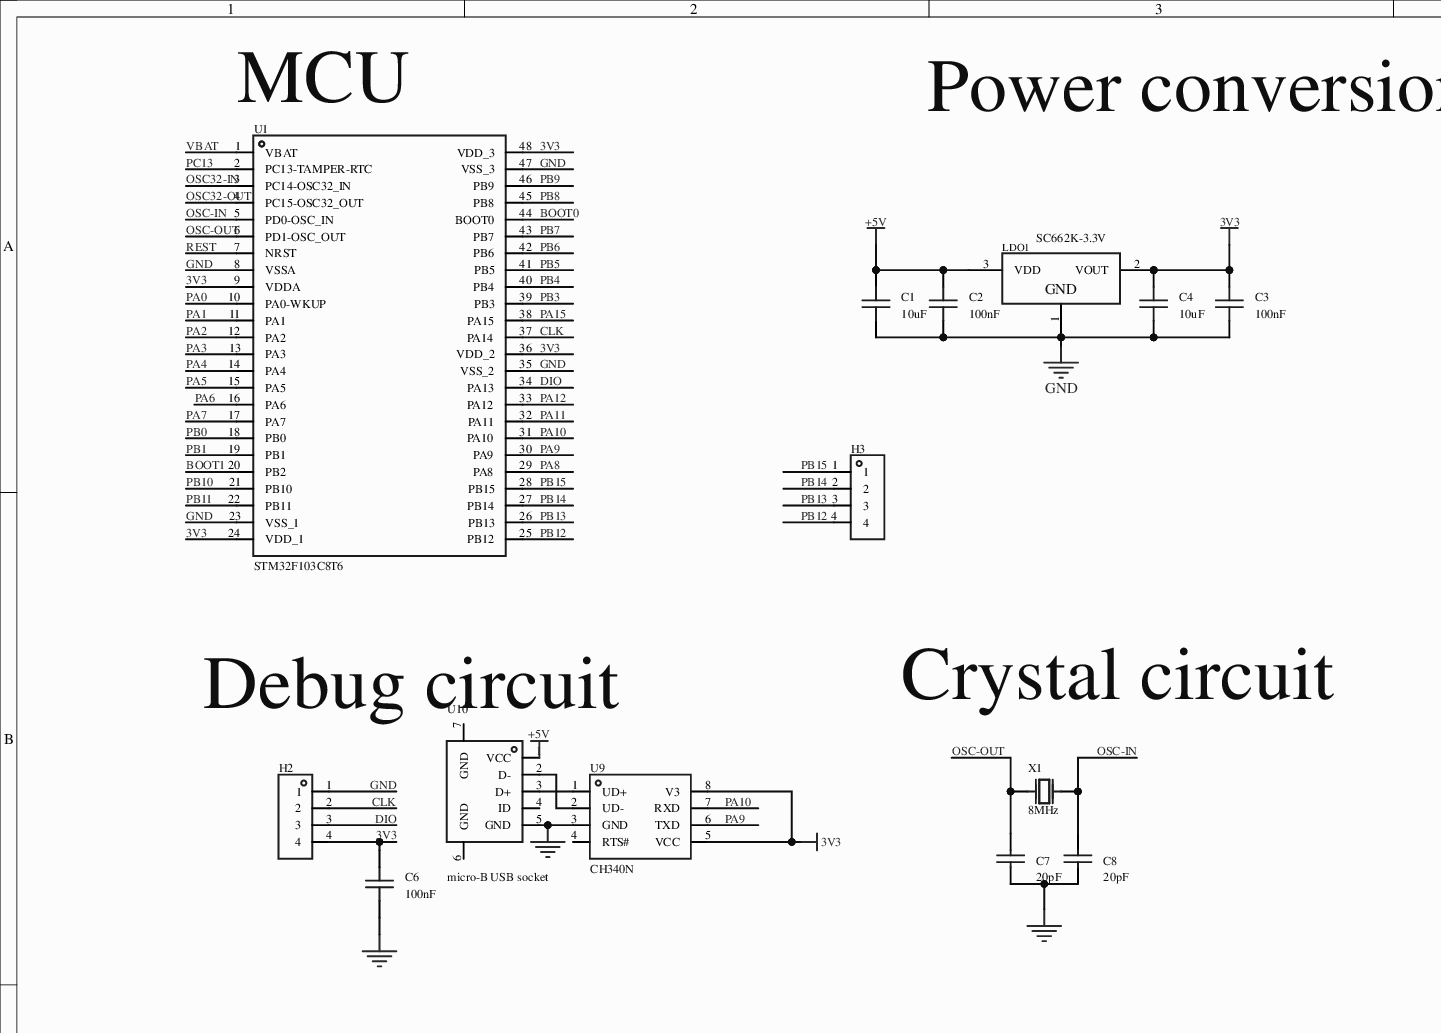
[diagram p0: MISC64779-3.schdoc, top left]
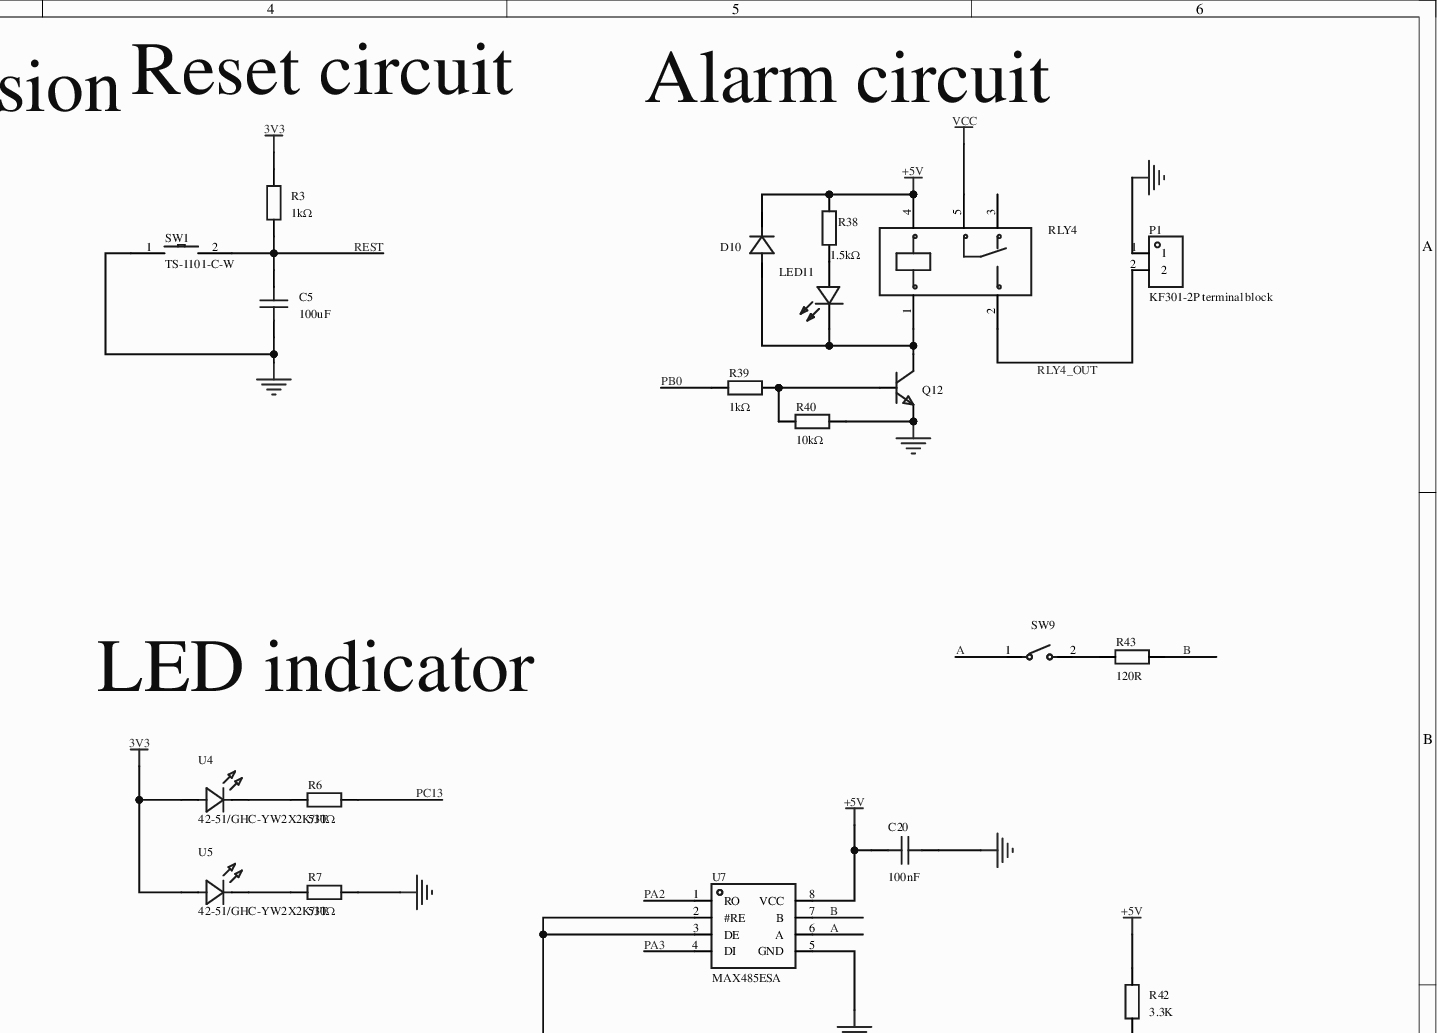
[diagram p1: MISC64779-3.schdoc, top right]
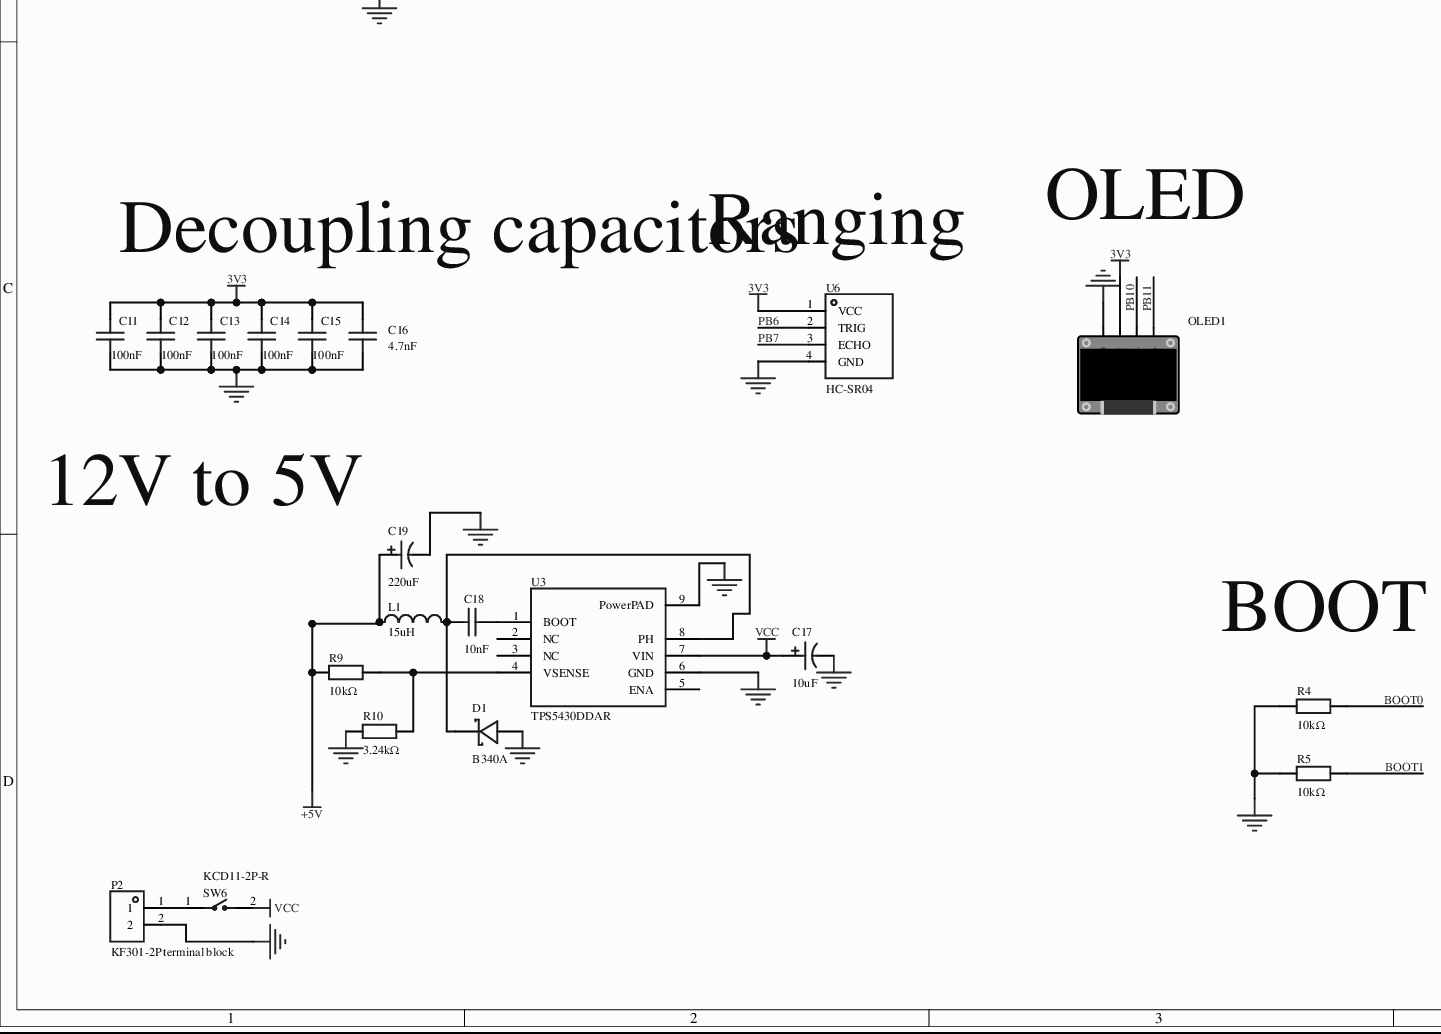
[diagram p2: MISC64779-3.schdoc, bottom left]
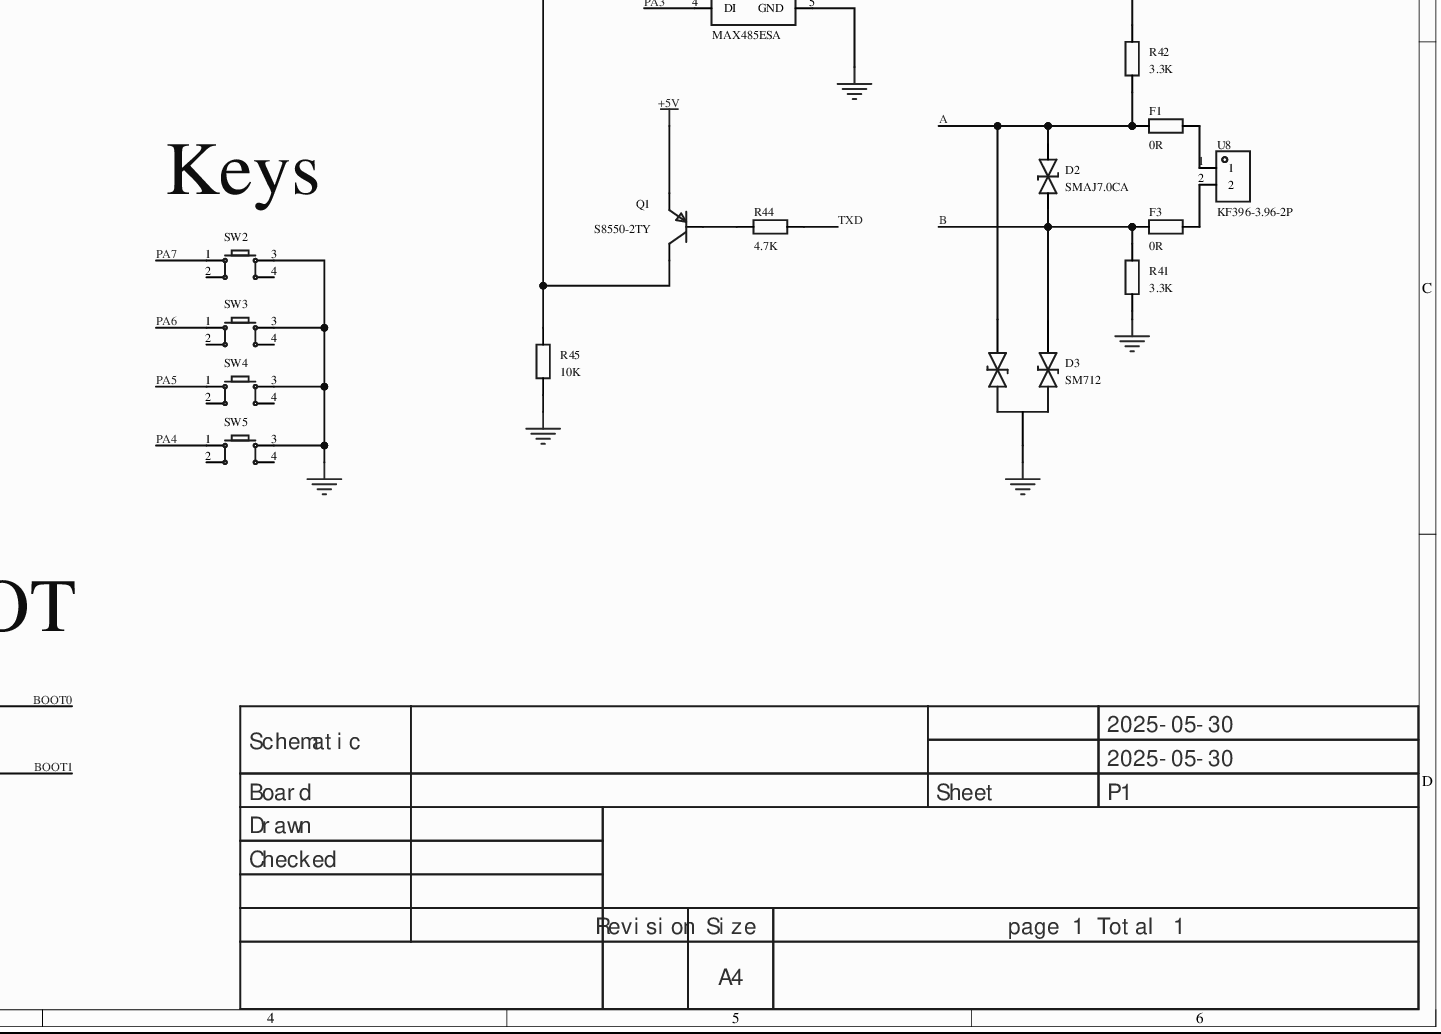
[diagram p3: MISC64779-3.schdoc, bottom right]
# Altium project MISC64779-2.PrjPcb
1 sheet, 67 parts. Net scope: global (net labels, ports and power ports of the same name join across sheets).
Board file: MISC64779.pcbdoc

## Sheet MISC64779-3.schdoc
size 420 x 297 mm; Version: V1.0; @Project Name: MISC64779; @Page Count: 1; @Update Date: 2025-05-30; @Create Date: 2025-05-30; @Schematic Name: MISC64779; @Page No: 1; @Create Time: 10:06:22; @Update Time: 12:30:53; @Board Name: MISC64779

### Parts
C1  10uF  [C0603]
C2  100nF  [C0603]
C3  100nF  [C0603]
C4  10uF  [C0603]
C5  100uF  [C1206]
C6  100nF  [C0603]
C7  20pF  [C0603]
C8  20pF  [C0603]
C11  100nF  [C0603]
C12  100nF  [C0603]
C13  100nF  [C0603]
C14  100nF  [C0603]
C15  100nF  [C0603]
C16  4.7nF  [C0603]
C17  10uF  [CAP-TH_BD5.0-P2.00-D0.8-FD]
C18  10nF  [C0603]
C19  220uF  [CAP-TH_BD6.3-P2.50-D1.0-FD]
C20  100nF  [C0603]
D1  B340A  [SMA_L4.3-W2.6-LS5.1-RD]
D2  SMAJ7.0CA  [SMA_L4.5-W2.7-LS5.1-BI]
D3  SM712  [SOT-23-3_L2.9-W1.3-P1.90-LS2.4-BR]
D10  1N4007  [SMA_L4.3-W2.5-LS5.0-RD]  (value not drawn)
F1  0R  [R0805]
F3  0R  [R0805]
H2  (no value)  [HDR-TH_4P-P2.54-V-M]
H3  (no value)  [HDR-TH_4P-P2.54-V-M]
L1  15uH  [IND-SMD_L7.0-W6.6_FXL0630]
LDO1  SC662K-3.3V  [SOT-23-3_L2.9-W1.3-P1.90-LS2.4-BR]
LED11  NCD0805R1  [LED0805-R-RD]  (value not drawn)
OLED1  (no value)  [0.96OLED_4P]
P1  KF301-2P terminal block  [CONN-TH_XY301V-A-5.0-2P]
P2  KF301-2P terminal block  [CONN-TH_XY301V-A-5.0-2P]
Q1  S8550-2TY  [SOT-23-3_L2.9-W1.3-P0.95-LS2.4-BR]
Q12  S8050 J3Y(RANGE:200-350)  [SOT-23-3_L3.0-W1.7-P0.95-LS2.9-BR]  (value not drawn)
R3  1kΩ  [R0603]
R4  10kΩ  [R0603]
R5  10kΩ  [R0603]
R6  510Ω  [R0603]
R7  510Ω  [R0603]
R9  10kΩ  [R0603]
R10  3.24kΩ  [R0603]
R38  1.5kΩ  [R0805]
R39  1kΩ  [R0805]
R40  10kΩ  [R0805]
R41  3.3K  [R0603]
R42  3.3K  [R0603]
R43  120R  [R0603]
R44  4.7K  [R0603]
R45  10K  [R0603]
RLY4  SRD-05VDC-SL-C  [RELAY-TH_SRD-XXVDC-XL-C]  (value not drawn)
SW1  TS-1101-C-W  [SW-SMD_L6.0-W3.3-LS8.0]
SW2  (no value)  [SW-TH_4P-L6.0-W6.0-P4.50-LS6.5]
SW3  (no value)  [SW-TH_4P-L6.0-W6.0-P4.50-LS6.5]
SW4  (no value)  [SW-TH_4P-L6.0-W6.0-P4.50-LS6.5]
SW5  (no value)  [SW-TH_4P-L6.0-W6.0-P4.50-LS6.5]
SW6  KCD11-2P-R  [SW-TH_2P-L15.0-W10.5-P5.00_KCD11-2P-R]
SW9  ZX-1.27BM-1PSMD  [SW-SMD_L5.4-W2.8-LS8.2]  (value not drawn)
U1  STM32F103C8T6  [LQFP-48_L7.0-W7.0-P0.50-LS9.0-BL]
U3  TPS5430DDAR  [ESOP-8_L4.9-W3.9-P1.27-LS6.0-TL-EP]
U4  42-51/GHC-YW2X2K/3T  [LED-SMD_L1.6-W0.8-FD_GREEN-1]
U5  42-51/GHC-YW2X2K/3T  [LED-SMD_L1.6-W0.8-FD_GREEN-1]
U6  HC-SR04  [TH_HC-SR04V]
U7  MAX485ESA  [SOP-8_L5.0-W4.0-P1.27-LS6.0-BL]
U8  KF396-3.96-2P  [CONN-TH_P3.96_KF396-3.96-2P]
U9  CH340N  [SOP-8_L4.9-W3.9-P1.27-LS6.0-BL]
U10  micro-B USB socket  [MICRO-USB_C9900039549]
X1  8MHz  [OSC-TH_L10.0-W4.5-P5.00]

### Nets
3V3: C3.2 C4.2 C6.2 C11.2 C12.2 C13.2 C14.2 C15.2 C16.2 H2.4 LDO1.2(VOUT) OLED1.2(VCC) R3.2 U1.9(VDDA) U1.24(VDD_1) U1.36(VDD_2) U1.48(VDD_3) U4.1(A) U5.1(A) U6.1(VCC) U9.5(VCC) U9.8(V3)
+5V: C1.2 C2.2 C19.1 C20.1 D10.1(K) L1.1 LDO1.3(VDD) Q1.2(E) R9.1 R38.2 R42.2 RLY4.4 U7.8(VCC) U10.1(VCC)
GND: C1.1 C2.1 C3.1 C4.1 C5.1 C6.1 C7.1 C8.1 C11.1 C12.1 C13.1 C14.1 C15.1 C16.1 C17.2 C19.2 C20.2 D1.2(A) D3.3 H2.1 LDO1.1(GND) OLED1.1(GND) P1.1 P2.2 Q12.2(E) R4.1 R5.1 R7.2 R10.1 R40.1 R41.1 R45.2 SW1.1 SW2.3 SW3.3 SW4.3 SW5.3 U1.8(VSSA) U1.23(VSS_1) U1.35(VSS_2) U1.47(VSS_3) U3.6(GND) U3.9(PowerPAD) U6.4(GND) U7.5(GND) U9.3(GND) U10.5(GND)
VCC: C17.1 RLY4.5 SW6.2 U3.7(VIN)
A: D2.2 D3.2 F1.1 R42.1 SW9.1 U7.6(A)
B: D2.1 D3.1 F3.1 R41.2 R43.2 U7.7(B)
BOOT0: R4.2 U1.44(BOOT0)
BOOT1: R5.2 U1.20(PB2)
CLK: H2.2 U1.37(PA14)
DIO: H2.3 U1.34(PA13)
OSC32-IN: U1.3(PC14-OSC32_IN)
OSC32-OUT: U1.4(PC15-OSC32_OUT)
OSC-IN: C8.2 U1.5(PD0-OSC_IN) X1.1(OSC1)
OSC-OUT: C7.2 U1.6(PD1-OSC_OUT) X1.2(OSC2)
PA0: U1.10(PA0-WKUP)
PA1: U1.11(PA1)
PA2: U1.12(PA2) U7.1(RO)
PA3: U1.13(PA3) U7.4(DI)
PA4: SW5.1 U1.14(PA4)
PA5: SW4.1 U1.15(PA5)
PA6: SW3.1 U1.16(PA6)
PA7: SW2.1 U1.17(PA7)
PA8: U1.29(PA8)
PA9: U1.30(PA9) U9.6(TXD)
PA10: U1.31(PA10) U9.7(RXD)
PA11: U1.32(PA11)
PA12: U1.33(PA12)
PA15: U1.38(PA15)
PB0: R39.1 U1.18(PB0)
PB1: U1.19(PB1)
PB3: U1.39(PB3)
PB4: U1.40(PB4)
PB5: U1.41(PB5)
PB6: U1.42(PB6) U6.2(TRIG)
PB7: U1.43(PB7) U6.3(ECHO)
PB8: U1.45(PB8)
PB9: U1.46(PB9)
PB10: OLED1.3(SCL) U1.21(PB10)
PB11: OLED1.4(SDA) U1.22(PB11)
PB12: H3.4 U1.25(PB12)
PB13: H3.3 U1.26(PB13)
PB14: H3.2 U1.27(PB14)
PB15: H3.1 U1.28(PB15)
PC13: R6.2 U1.2(PC13-TAMPER-RTC)
REST: C5.2 R3.1 SW1.2 U1.7(NRST)
RLY4_OUT: P1.2 RLY4.2
TXD: R44.1
VBAT: U1.1(VBAT)
NetC18_1: C18.1 D1.1(K) L1.2 U3.8(PH)
NetC18_2: C18.2 U3.1(BOOT)
NetD10_2: D10.2(A) LED11.2(-) Q12.3(C) RLY4.1
NetF1_2: F1.2 U8.1
NetF3_2: F3.2 U8.2
NetLED11_1: LED11.1(+) R38.1
NetP2_1: P2.1 SW6.1
NetQ1_1: Q1.1(B) R44.2
NetQ1_3: Q1.3(C) R45.1 U7.2(#RE) U7.3(DE)
NetQ12_1: Q12.1(B) R39.2 R40.2
NetR6_1: R6.1 U4.2(C)
NetR7_1: R7.1 U5.2(C)
NetR9_2: R9.2 R10.2 U3.4(VSENSE)
NetR43_1: R43.1 SW9.2
NetU9_1: U9.1(UD+) U10.3(D+)
NetU9_2: U9.2(UD-) U10.2(D-)

Not connected (* = marked no-connect by the designer): RLY4 3*; SW2 2 4; SW3 2 4; SW4 2 4; SW5 2 4; U3 2(NC) 3(NC) 5(ENA); U9 4(RTS#); U10 4(ID) 6(GND) 7(GND)

### Notes on the sheet
- (near U1) MCU
- Power conversion
- Reset circuit
- Alarm circuit
- 供电用12v供电
  有超声波测距功能
  具备连接上位机的功能
  有报警功能（留接口）
  用户按键，LED
  温湿度，oled显示
- (near U10) Debug circuit
- Crystal circuit
- LED indicator
- (near SW2) Keys
- Decoupling capacitors
- (near U6) Ranging
- OLED
- (near C19) 12V to 5V
- (near R4) BOOT
- 2025-05-30
- Schematic
- Board
- Sheet
- P1
- Drawn
- Checked
- Revision
- Size
- A4
- page 1 Total 1

### Library data of the parts
C1 C4 = CL10A106KP8NNNC: Capacitance:10uF;Tolerance:±10%;Rated voltage:10V;Dielectric (temp. coefficient):X5R;; Manufacturer: SAMSUNG(三星); AddInBom: yes; ModelId: ac125912035d415993ca9572d50418b1; ModelName: C0603_L1.6-W0.8-H0.8; ModelTransform: 62.992,31.496,0,0,0,0,0,0,0; Tolerance: ±10%; Voltage Rated: 10V; Temperature Coefficient: X5R; Device: CL10A106KP8NNNC; Symbol: CL10A106KP8NNNC; LCSC Part Name: 10uF ±10% 10V; SupplierPart: C19702; ManufacturerPart: CL10A106KP8NNNC; Supplier Footprint: 0603; JLCPCB Part Class: Basic library; Datasheet: example.com/20160103/1457707703378.pdf; Supplier: LCSC; ConvertToPcb: yes; FootprintName: C0603; Value: 10uF
C2 C3 = CC0603KRX7R9BB104: Capacitance:100nF;Tolerance:±10%;Rated voltage:50V;Dielectric (temp. coefficient):X7R;; Manufacturer: YAGEO(国巨); AddInBom: yes; ModelId: ac125912035d415993ca9572d50418b1; ModelName: C0603_L1.6-W0.8-H0.8; ModelTransform: 62.992,31.496,0,0,0,0,0,0,0; Tolerance: ±10%; Voltage Rated: 50V; Temperature Coefficient: X7R; Device: CC0603KRX7R9BB104; Symbol: CC0603KRX7R9BB104; LCSC Part Name: 100nF ±10% 50V; SupplierPart: C14663; ManufacturerPart: CC0603KRX7R9BB104; Supplier Footprint: 0603; JLCPCB Part Class: Basic library; Datasheet: example.com/20180910/C282072_33301C7F631E79921B82A8DAC6BCC5B3.pdf; Supplier: LCSC; ConvertToPcb: yes; FootprintName: C0603; Value: 100nF
C5 = HGC1206R5107M100NSPJ: Capacitance:100uF;Tolerance:±20%;Rated voltage:10V;Dielectric (temp. coefficient):X5R;; Manufacturer: Chinocera(华瓷); AddInBom: yes; ModelId: e4be705b945545a48e666415e3682bd8; ModelName: C1206_L3.2-W1.6-H1.3; ModelTransform: 125.984,62.992,0,0,0,0,0,0,0; Tolerance: ±20%; Voltage Rated: 10V; Temperature Coefficient: X5R; Symbol: HGC1206R5107M100NSPJ; Device: HGC1206R5107M100NSPJ; LCSC Part Name: 100uF ±20% 10V; SupplierPart: C7432784; ManufacturerPart: HGC1206R5107M100NSPJ; Supplier Footprint: 1206; JLCPCB Part Class: Extended library; Datasheet: example.com/20240320/FAC3FEC40A78BC5CCCE96C232A94D860.pdf; Supplier: LCSC; ConvertToPcb: yes; FootprintName: C1206; Value: 100uF
C6 C11-C15 = CGA0603X7R104K500JT: Capacitance:100nF;Tolerance:±10%;Rated voltage:50V;Dielectric (temp. coefficient):X7R;; Manufacturer: HRE(芯声); AddInBom: yes; ModelId: ac125912035d415993ca9572d50418b1; ModelName: C0603_L1.6-W0.8-H0.8; ModelTransform: 62.992,31.496,0,0,0,0,0,0,0; Tolerance: ±10%; Voltage Rated: 50V; Temperature Coefficient: X7R; Symbol: CGA0603X7R104K500JT; Device: CGA0603X7R104K500JT; LCSC Part Name: 100nF ±10% 50V; SupplierPart: C6119867; ManufacturerPart: CGA0603X7R104K500JT; Supplier Footprint: 0603; JLCPCB Part Class: Extended library; Supplier: LCSC; ConvertToPcb: yes; FootprintName: C0603; Value: 100nF
C7 C8 = CL10C200JB8NNNC: Capacitance:20pF;Tolerance:±5%;Rated voltage:50V;Dielectric (temp. coefficient):C0G;; Manufacturer: SAMSUNG(三星); AddInBom: yes; ModelId: ac125912035d415993ca9572d50418b1; ModelName: C0603_L1.6-W0.8-H0.8; ModelTransform: 62.992,31.496,0,0,0,0,0,0,0; Tolerance: ±5%; Voltage Rated: 50V; Temperature Coefficient: C0G; Symbol: CL10C200JB8NNNC; Device: CL10C200JB8NNNC; LCSC Part Name: 20pF ±5% 50V; SupplierPart: C1648; ManufacturerPart: CL10C200JB8NNNC; Supplier Footprint: 0603; JLCPCB Part Class: Basic library; Datasheet: example.com/20160218/1457707763339.pdf; Supplier: LCSC; ConvertToPcb: yes; FootprintName: C0603; Value: 20pF
C16 = CGA0603X7R472K500JT: Capacitance:4.7nF;Tolerance:±10%;Rated voltage:50V;Dielectric (temp. coefficient):X7R;; Manufacturer: HRE(芯声); AddInBom: yes; ModelId: ac125912035d415993ca9572d50418b1; ModelName: C0603_L1.6-W0.8-H0.8; ModelTransform: 62.992,31.496,0,0,0,0,0,0,0; Tolerance: ±10%; Voltage Rated: 50V; Temperature Coefficient: X7R; Symbol: CGA0603X7R472K500JT; Device: CGA0603X7R472K500JT; LCSC Part Name: 4.7nF ±10% 50V; SupplierPart: C7503499; ManufacturerPart: CGA0603X7R472K500JT; Supplier Footprint: 0603; JLCPCB Part Class: Extended library; Supplier: LCSC; ConvertToPcb: yes; FootprintName: C0603; Value: 4.7nF
C17 = KM106M050D11RR0VH2FP0: Capacitance:10uF;Tolerance:±20%;Rated voltage:50V;; Manufacturer: CX(承兴); Symbol: 10uF 50V 5*11; AddInBom: yes; ModelId: edeeed87cbc746108d01291548c38636; ModelName: CAP-TH_D5.0×H7.0×P2.0; ModelTransform: 197.091,196.7911,0,0,0,0,0,0,-137.795; Tolerance: ±20%; Rated Voltage: 50V; φD: 5mm; L: 11mm; Lifetime @ Temp: 1000hrs@105℃; Device: KM106M050D11RR0VH2FP0; Supplier: LCSC; Manufacturer Part: KM106M050D11RR0VH2FP0; Value: 10uF; Supplier Part: C43345; JLCPCB Part Class: Extended library; LCSC Part Name: 10uF ±20% 50V; Supplier Footprint: 插件,D5xL11mm; Datasheet: example.com/20211027/06D6BA3719C264B639DC286D935D03EA.pdf; ConvertToPcb: yes; FootprintName: CAP-TH_BD5.0-P2.00-D0.8-FD; Lead Spacing: 2mm
C18 = CC0603KRX7R9BB103: Capacitance:10nF;Tolerance:±10%;Rated voltage:50V;Dielectric (temp. coefficient):X7R;; Manufacturer: YAGEO(国巨); AddInBom: yes; ModelId: ac125912035d415993ca9572d50418b1; ModelName: C0603_L1.6-W0.8-H0.8; ModelTransform: 62.992,31.496,0,0,0,0,0,0,0; Tolerance: ±10%; Voltage Rated: 50V; Temperature Coefficient: X7R; Symbol: CC0603KRX7R9BB103; Device: CC0603KRX7R9BB103; Supplier: LCSC; Manufacturer Part: CC0603KRX7R9BB103; Value: 10nF; Supplier Part: C100042; JLCPCB Part Class: Extended library; LCSC Part Name: 10nF ±10% 50V; Supplier Footprint: 0603; Datasheet: example.com/20181008/C309510_22F155564471FAF6A489F7D68F34234E.pdf; ConvertToPcb: yes; FootprintName: C0603
C19 = KM227M016E11RR0VH2FP0: Capacitance:220uF;Tolerance:±20%;Rated voltage:16V;Ripple current:-;Equivalent series resistance:-;; Manufacturer: CX(承兴); Symbol: 220uF 16V 6.3*11; AddInBom: yes; ModelId: 0a4db4bf24b443b3be4905be97ff10c5; ModelTransform: 248.4247,247.99777,0,0,0,0,0,0,-137.795; Tolerance: ±20%; Rated Voltage: 16V; φD: 6.3mm; L: 11mm; Lifetime @ Temp: 1000hrs@105℃; Device: KM227M016E11RR0VH2FP0; Supplier: LCSC; Manufacturer Part: KM227M016E11RR0VH2FP0; Value: 220uF; Supplier Part: C43349; JLCPCB Part Class: Extended library; LCSC Part Name: 220uF ±20% 16V; Supplier Footprint: 插件,D6.3xL11mm; Datasheet: example.com/20211027/06D6BA3719C264B639DC286D935D03EA.pdf; ConvertToPcb: yes; FootprintName: CAP-TH_BD6.3-P2.50-D1.0-FD; ModelName: CAP-TH_BD6.3-P2.50-D1.0-FD; Ripple Current: -; Equivalent Series Resistance(ESR): -; Lead Spacing: 2.5mm
C20 = CAP_0603: ConvertToPcb: yes; SymbolName: CapAcitance; ModelId: ac125912035d415993ca9572d50418b1; ModelName: C0603_L1.6-W0.8-H0.8; ModelTransform: 62.992,31.496,0,0,0,0,0,0,0; Device: CAP_0603; AddInBom: yes; Supplier Footprint: 0603; FootprintName: C0603; Value: 100nF
D1 = B340A: Forward voltage drop (Vf):550mV@3A;DC reverse voltage (Vr):40V;Average rectified current (Io):3A;; Manufacturer: MDD; AddInBom: yes; ModelId: 1d20a911e9694ba6aaf6e9207164e4da; ModelTransform: 196.4563,102.362,0,0,0,0,0,0,0; Reverse Voltage (Vr): 40V; Average Rectified Current (Io): 3A; Symbol: B340A; Device: B340A; Supplier: LCSC; Manufacturer Part: B340A; Supplier Part: C64982; JLCPCB Part Class: Extended library; LCSC Part Name: 电压:40V 电流:3A; Supplier Footprint: SMA(DO-214AC); Datasheet: example.com/20230710/CC7CF81239BC87A7012E02A96905E83C.pdf; ConvertToPcb: yes; FootprintName: SMA_L4.3-W2.6-LS5.1-RD; ModelName: SMA_L4.3-W2.6-LS5.1-RD; Forward Voltage (Vf@If): 550mV@3A
D2 = SMAJ7.0CA_C383701: Reverse standoff voltage (Vrwm):7V;Max clamping voltage:12V;Peak pulse current (Ipp)@10/1000us:33.3A;Breakdown voltage:7.78V;; Manufacturer: BORN(伯恩半导体); AddInBom: yes; ModelId: c57f874422f846fca512c5458c0e414d; ModelTransform: 200.787,106.299,0,0,0,0,0,0,0; Reverse Stand-Off Voltage (Vrwm): 7V; Maximum Clamping Voltage: 12V; Peak Pulse Current (Ipp)@10/1000us: 33.3A; Breakdown Voltage: 7.78V; Type: TVS; Symbol: SMAJ7.0CA_C383701; Device: SMAJ7.0CA_C383701; Supplier: LCSC; Supplier Part: C383701; Manufacturer Part: SMAJ7.0CA; JLCPCB Part Class: Extended library; LCSC Part Name: SMAJ7.0CA; Supplier Footprint: SMA(DO-214AC); Datasheet: example.com/20190401/C383701_4E66D368F6F089B11959B32E4033EF5C.pdf; ConvertToPcb: yes; FootprintName: SMA_L4.5-W2.7-LS5.1-BI; ModelName: SMA_L4.5-W2.7-LS5.1-BI
D3 = SM712_C521963: eak Pulse Current ( tp =8/20μs ) (note1) IPP 17A，反向截断电压VRWM 7V+12V 反向漏泄电流IR=1μA，VC12V 17A=26V VC7V 17A=12V 结电容75PF; Manufacturer: TECH PUBLIC(台舟); AddInBom: yes; ModelId: c62791f0466c4ae2a892c056b845b0ca; ModelName: SOT-23-3P_L2.9-W1.3-H1.0-LS2.4-P0.95; ModelTransform: 98.425,114.173,0,180,0,0,0.0005,-0.0005,0; Symbol: SM712_C521963; Device: SM712_C521963; Supplier: LCSC; Supplier Part: C521963; Manufacturer Part: SM712; JLCPCB Part Class: Extended library; LCSC Part Name: SM712; Supplier Footprint: SOT-23; Datasheet: example.com/20210810/E76C7C1824B0CB2A5B8963B3ABCE2DCE.pdf; ConvertToPcb: yes; FootprintName: SOT-23-3_L2.9-W1.3-P1.90-LS2.4-BR
D10 = 1N4007_C727081: Diode configuration:Single;Forward voltage drop (Vf):1.1V@1A;DC reverse voltage (Vr):1kV;Rectified current:1A;; Manufacturer: TWGMC(台湾迪嘉); AddInBom: yes; ModelId: 5b53cc1b87a148cc9fa13125be89f948; ModelTransform: 194.8815,98.425,0,0,0,0,0,0,0; Diode Configuration: Single; Reverse Voltage (Vr): 1kV; Rectified Current: 1A; Reverse Leakage Current (Ir): 5uA; Symbol: 1N4007_C727081; Device: 1N4007_C727081; LCSC Part Name: 1N4007; SupplierPart: C727081; ManufacturerPart: 1N4007; Supplier Footprint: SMA(DO-214AC); JLCPCB Part Class: Extended library; Datasheet: example.com/20200828/C727079_3A05254382567072883400655AE0ED46.pdf; Supplier: LCSC; ConvertToPcb: yes; FootprintName: SMA_L4.3-W2.5-LS5.0-RD; ModelName: SMA_L4.3-W2.5-LS5.0-RD; Forward Voltage (Vf@If): 1.1V@1A
F1 F3 = Res_0805: Symbol: Resistor; ConvertToPcb: yes; ModelId: 37a81e68749a4138bd2dfa6897b24b85; ModelName: R0805_L2.0-W1.3-H0.6; ModelTransform: 78.74,51.181,0,0,0,0,0,-0.0005,0; Value: 0R; Device: Res_0805; AddInBom: yes; Supplier Footprint: 0805; FootprintName: R0805
H2 H3 = HDR-M_2.54_1x4P: Symbol: PZ254V-11-04P; ConvertToPcb: yes; ModelId: 112f4d05e8d64e99ab9a333894bea4f9; ModelName: HDR-TH_4P-P2.54-M-LI-1X4P; ModelTransform: 399.999,104.7242,0,0,0,0,0,0,-118.11; Device: HDR-M_2.54_1x4P; AddInBom: yes; SupplierPart: C492403; Supplier Footprint: 插件; FootprintName: HDR-TH_4P-P2.54-V-M
L1 = FXL0630-150-M: Inductance:15uH;Tolerance:±20%;Rated current:3A;Saturation current (Isat):4.5A;Type:Integrally molded inductor;; Manufacturer: cjiang(长江微电); AddInBom: yes; ModelId: 6712504104d74f0ca01cd7d0df9965b7; ModelName: IND-SMD_L7.0-W6.6-H2.8_FXL0630; ModelTransform: 275.59,259.842,0,0,0,0,0,0,0; Tolerance: ±20%; Rated Current: 3A; Saturation Current (Isat): 4.5A; DC Resistance (DCR): 115mΩ; Symbol: FXL0630-150-M; Device: FXL0630-150-M; LCSC Part Name: 15uH ±20% 4.5A; SupplierPart: C177243; ManufacturerPart: FXL0630-150-M; Supplier Footprint: SMD,6.6x7mm; JLCPCB Part Class: Extended library; Datasheet: example.com/20230516/3A080F5AF8C87BB81C3BA86E5F60E51A.pdf; Supplier: LCSC; ConvertToPcb: yes; FootprintName: IND-SMD_L7.0-W6.6_FXL0630; Value: 15uH; Type: Integrally molded inductor
LDO1 = SC662K-3.3V: Output type:Fixed;Output polarity:Positive;Max input voltage:6V;Output voltage:3.3V;Output current:250mA;Power supply ripple rejection (PSRR):50dB@(1kHz);; Manufacturer: FM(富满); AddInBom: yes; ModelId: c62791f0466c4ae2a892c056b845b0ca; ModelName: SOT-23-3P_L2.9-W1.3-H1.0-LS2.4-P0.95; ModelTransform: 98.425,114.173,0,180,0,0,0.0005,-0.0005,0; Output Type: Fixed; Number of Outputs: 1; Maximum Input Voltage: 6V; Output Voltage: 3.3V; Dropout Voltage: 38mV@(10mA); Output Current: 250mA; Symbol: SC662K-3.3V; Device: SC662K-3.3V; Supplier: LCSC; Manufacturer Part: SC662K-3.3V; Supplier Part: C83932; JLCPCB Part Class: Extended library; LCSC Part Name: 输入6V 输出3.3V 250mA 停产; Supplier Footprint: SOT-23; Datasheet: example.com/20161024/1477288576049.pdf; ConvertToPcb: yes; FootprintName: SOT-23-3_L2.9-W1.3-P1.90-LS2.4-BR; Output Polarity: Positive; Power Supply Rejection Ratio (PSRR): 50dB@(1kHz)
LED11 = NCD0805R1: 灯头类型:-;发光颜色:红色;正向电压(VF):1.6V~2.6V;功率:65mW;正向电流:20mA;主波长:615nm~630nm;二极管配置:独立二极管;透镜颜色:无色透明透镜;色温:-;发光强度:67mcd~195mcd;发光角度:130°;载带方式:-;工作温度:-30℃~+85℃;; Manufacturer: 国星光电; Symbol: FC-2012HRK-620D; AddInBom: yes; ModelId: 6ccd75a2b5134d6ab756ecf3c14a7290; ModelName: LED0805-RD; ModelTransform: 79.527,49.2125,0,0,0,0,0,0,0; Emitted Color: Red; Power Dissipation: 65mW; Forward Current: 20mA; Diode Configuration: Single diode; Lens Color: Clear lens; Viewing Angle: 130°; Device: NCD0805R1; LCSC Part Name: NCD0805R1; SupplierPart: C84256; ManufacturerPart: NCD0805R1; Supplier Footprint: 0805; JLCPCB Part Class: Basic library; Datasheet: example.com/20200820/C84256_F0A75A43B3EAD75808600A0514C76B99.pdf; Supplier: LCSC; ConvertToPcb: yes; FootprintName: LED0805-R-RD; Lamp Holder Type: -; Forward Voltage (VF): 1.6V~2.6V; Dominant Wavelength: 615nm~630nm; Peak Wavelength: -; Color Temperature: -; Luminous Intensity: 67mcd~195mcd; Mounting Sytle: -; Operating Temperature: -30℃~+85℃
OLED1 = 0.96OLED模块_4P: Device: 0.96OLED module_4P; ConvertToPcb: yes; ModelId: 79c000fdb68d45a296c2e9bedf4f9055; ModelTransform: 1393.69792,1318.895,0,0,0,0,0,-560.079,-137.795; AddInBom: yes; SymbolName: 0.96OLED module_4P; FootprintName: 0.96OLED_4P; Supplier Footprint: 插件; ModelName: 0.96OLED_4P
P1 P2 = KF301-2P接线端子: AddInBom: yes; ModelId: ef7ead88b0f2448d904975b26718870f; ModelTransform: 417.322,299.212,0,0,0,0,11.811,-7.835,-157.48; Symbol: KF301-2P terminal block; Device: KF301-2P terminal block; LCSC Part Name: KF301-2P接线端子; SupplierPart: C9900016950; ManufacturerPart: KF301-2P接线端子; Supplier Footprint: CK301-2P; JLCPCB Part Class: Extended library; Supplier: LCSC; ConvertToPcb: yes; FootprintName: CONN-TH_XY301V-A-5.0-2P; ModelName: CONN-TH_XY301V-A-5.0-2P
Q1 = S8550-2TY: Transistor type:PNP;Collector current (Ic):1.5A;Collector-emitter breakdown voltage (Vceo):25V;Power (Pd):300mW;; Manufacturer: MDD; AddInBom: yes; ModelId: c62791f0466c4ae2a892c056b845b0ca; ModelName: SOT-23-3P_L2.9-W1.3-H1.0-LS2.4-P0.95; ModelTransform: 98.425,114.173,0,180,0,0,0.0005,-0.0005,0; Transistor Type: PNP; Collector Current (Ic): 1.5A; Collector-Emitter Breakdown Voltage (Vceo): 25V; Power Dissipation (Pd): 300mW; Transition Frequency (fT): 100MHz; Collector Cut-Off Current (Icbo): 100nA; Collector-Emitter Saturation Voltage (VCE(sat)@Ic,Ib): 500mV@800mA,80mA; Symbol: S8550-2TY; Device: S8550-2TY; Supplier: LCSC; Supplier Part: C364313; Manufacturer Part: S8550-2TY; JLCPCB Part Class: Extended library; LCSC Part Name: PNP 电流:1.5A 耐压:25V; Supplier Footprint: SOT-23; Datasheet: example.com/20230823/1A247BF48B2A25A14EBA2E9BB5B5D25C.pdf; ConvertToPcb: yes; FootprintName: SOT-23-3_L2.9-W1.3-P0.95-LS2.4-BR; Operating Temperature: -
Q12 = S8050 J3Y(RANGE:200-350): Transistor type:NPN;Collector current (Ic):500mA;Collector-emitter breakdown voltage (Vceo):25V;Power dissipation (Pd):300mW;DC current gain (hFE):200@500mA,1V;; Manufacturer: CJ(江苏长电/长晶); Symbol: S8050_C2146; AddInBom: yes; ModelId: 89cb27a44ab2466697082bb9fd73a7d0; ModelName: SOT-23-3L_L2.9-W1.6-H1.1-LS2.8-P0.95; ModelTransform: 114.173,110.236,0,90,0,0,0,0,0; type: NPN; Current - Collector(Ic): 500mA; Collector - Emitter Voltage VCEO: 25V; Pd - Power Dissipation: 300mW; Transition frequency(fT): 150MHz; Current - Collector Cutoff: 100nA; Vce Saturation(VCE(sat)): 600mV; Device: S8050 J3Y(RANGE:200-350); LCSC Part Name: H档(200-350); SupplierPart: C2146; ManufacturerPart: S8050 J3Y(RANGE:200-350); Supplier Footprint: SOT-23; JLCPCB Part Class: Basic library; Datasheet: example.com/20231013/FF37B6A000E6CDA75C9C999D2E78731F.pdf; Supplier: LCSC; ConvertToPcb: yes; FootprintName: SOT-23-3_L3.0-W1.7-P0.95-LS2.9-BR; DC Current Gain: 200@500mA,1V; Operating Temperature: -55℃~+150℃
R3 = RC0603FR-071KL: Resistor type:Thick-film resistor;Resistance:1kΩ;Tolerance:±1%;Power:100mW;Max working voltage:75V;Temperature coefficient:±100ppm/℃;; Manufacturer: YAGEO(国巨); AddInBom: yes; ModelId: fc143cca1e79419f9cd78b61e9279f08; ModelTransform: 31.8897,63.7794,0,90,0,0,0,0,0; Tolerance: ±1%; Power(Watts): 100mW; Overload Voltage (Max): 75V; Symbol: RC0603FR-071KL; Device: RC0603FR-071KL; LCSC Part Name: 厚膜电阻 1kΩ ±1% 100mW; SupplierPart: C22548; ManufacturerPart: RC0603FR-071KL; Supplier Footprint: 0603; JLCPCB Part Class: Extended library; Datasheet: example.com/20180316/70C0E2BDAE7FCC62C531A5A58D202EE1.pdf; Supplier: LCSC; ConvertToPcb: yes; FootprintName: R0603; ModelName: R0603; Type: Thick-film resistor; Value: 1kΩ; Temperature Coefficient: ±100ppm/℃; Operating Temperature Range: -55℃~+155℃
R4 R5 R9 = 0603WAF1002T5E: Resistor type:Thick-film resistor;Resistance:10kΩ;Tolerance:±1%;Power:100mW;Max working voltage:75V;Temperature coefficient:±100ppm/℃;; Manufacturer: UNI-ROYAL(厚声); AddInBom: yes; ModelId: fc143cca1e79419f9cd78b61e9279f08; ModelTransform: 31.8897,63.7794,0,90,0,0,0,0,0; Tolerance: ±1%; Power(Watts): 100mW; Overload Voltage (Max): 75V; Symbol: 0603WAF1002T5E; Device: 0603WAF1002T5E; LCSC Part Name: 厚膜电阻 10kΩ ±1% 100mW; SupplierPart: C25804; ManufacturerPart: 0603WAF1002T5E; Supplier Footprint: 0603; JLCPCB Part Class: Basic library; Datasheet: example.com/20200306/C422600_1E6D84923E4A46A82E41ADD87F860B5C.pdf; Supplier: LCSC; ConvertToPcb: yes; FootprintName: R0603; ModelName: R0603; Type: Thick-film resistor; Value: 10kΩ; Temperature Coefficient: ±100ppm/℃; Operating Temperature Range: -55℃~+155℃
R6 R7 = 0603WAF5100T5E: Resistor type:Thick-film resistor;Resistance:510Ω;Tolerance:±1%;Power:100mW;Max working voltage:75V;Temperature coefficient:±100ppm/℃;; Manufacturer: UNI-ROYAL(厚声); AddInBom: yes; ModelId: fc143cca1e79419f9cd78b61e9279f08; ModelTransform: 31.8897,63.7794,0,90,0,0,0,0,0; Tolerance: ±1%; Power(Watts): 100mW; Overload Voltage (Max): 75V; Symbol: 0603WAF5100T5E; Device: 0603WAF5100T5E; LCSC Part Name: 510Ω ±1% 100mW 厚膜电阻; SupplierPart: C23193; ManufacturerPart: 0603WAF5100T5E; Supplier Footprint: 0603; JLCPCB Part Class: Basic library; Datasheet: example.com/20200306/C422600_1E6D84923E4A46A82E41ADD87F860B5C.pdf; Supplier: LCSC; ConvertToPcb: yes; FootprintName: R0603; ModelName: R0603; Type: Thick-film resistor; Value: 510Ω; Temperature Coefficient: ±100ppm/℃; Operating Temperature Range: -55℃~+155℃
R10 = 0603WAF3241T5E: Resistor type:Thick-film resistor;Resistance:3.24kΩ;Tolerance:±1%;Power:100mW;Max working voltage:75V;Temperature coefficient:±100ppm/℃;; Manufacturer: UNI-ROYAL(厚声); AddInBom: yes; ModelId: fc143cca1e79419f9cd78b61e9279f08; ModelTransform: 31.8897,63.7794,0,90,0,0,0,0,0; Tolerance: ±1%; Power(Watts): 100mW; Overload Voltage (Max): 75V; Symbol: 0603WAF3241T5E; Device: 0603WAF3241T5E; LCSC Part Name: 3.24kΩ ±1% 100mW 厚膜电阻; SupplierPart: C22994; ManufacturerPart: 0603WAF3241T5E; Supplier Footprint: 0603; JLCPCB Part Class: Extended library; Datasheet: example.com/20200306/C422600_1E6D84923E4A46A82E41ADD87F860B5C.pdf; Supplier: LCSC; ConvertToPcb: yes; FootprintName: R0603; ModelName: R0603; Type: Thick-film resistor; Value: 3.24kΩ; Temperature Coefficient: ±100ppm/℃; Operating Temperature Range: -55℃~+155℃
R38 = 0805W8F1501T5E: Resistor type:Thick-film resistor;Resistance:1.5kΩ;Tolerance:±1%;Power:125mW;Max working voltage:150V;Temperature coefficient:±100ppm/℃;; Manufacturer: UNI-ROYAL(厚声); AddInBom: yes; ModelId: 37a81e68749a4138bd2dfa6897b24b85; ModelName: R0805_L2.0-W1.3-H0.6; ModelTransform: 78.74,51.181,0,0,0,0,0,-0.0005,0; Tolerance: ±1%; Power(Watts): 125mW; Overload Voltage (Max): 150V; Symbol: 0805W8F1501T5E; Device: 0805W8F1501T5E; LCSC Part Name: 1.5kΩ ±1% 125mW 厚膜电阻; SupplierPart: C4310; ManufacturerPart: 0805W8F1501T5E; Supplier Footprint: 0805; JLCPCB Part Class: Basic library; Datasheet: example.com/20200306/C422600_1E6D84923E4A46A82E41ADD87F860B5C.pdf; Supplier: LCSC; ConvertToPcb: yes; FootprintName: R0805; Type: Thick-film resistor; Value: 1.5kΩ; Temperature Coefficient: ±100ppm/℃; Operating Temperature Range: -55℃~+155℃
R39 = 0805W8F1001T5E: Resistor type:Thick-film resistor;Resistance:1kΩ;Tolerance:±1%;Power:125mW;Max working voltage:150V;Temperature coefficient:±100ppm/℃;; Manufacturer: UNI-ROYAL(厚声); AddInBom: yes; ModelId: 37a81e68749a4138bd2dfa6897b24b85; ModelName: R0805_L2.0-W1.3-H0.6; ModelTransform: 78.74,51.181,0,0,0,0,0,-0.0005,0; Tolerance: ±1%; Power(Watts): 125mW; Overload Voltage (Max): 150V; Symbol: 0805W8F1001T5E; Device: 0805W8F1001T5E; LCSC Part Name: 1kΩ ±1% 125mW 厚膜电阻; SupplierPart: C17513; ManufacturerPart: 0805W8F1001T5E; Supplier Footprint: 0805; JLCPCB Part Class: Basic library; Datasheet: example.com/20200306/C422600_1E6D84923E4A46A82E41ADD87F860B5C.pdf; Supplier: LCSC; ConvertToPcb: yes; FootprintName: R0805; Type: Thick-film resistor; Value: 1kΩ; Temperature Coefficient: ±100ppm/℃; Operating Temperature Range: -55℃~+155℃
R40 = 0805W8F1002T5E_C17414: Resistor type:Thick-film resistor;Resistance:10kΩ;Tolerance:±1%;Power:125mW;Max working voltage:150V;Temperature coefficient:±100ppm/℃;; Manufacturer: UNI-ROYAL(厚声); AddInBom: yes; ModelId: 37a81e68749a4138bd2dfa6897b24b85; ModelName: R0805_L2.0-W1.3-H0.6; ModelTransform: 78.74,51.181,0,0,0,0,0,-0.0005,0; Tolerance: ±1%; Power(Watts): 125mW; Overload Voltage (Max): 150V; Symbol: 0805W8F1002T5E; Device: 0805W8F1002T5E_C17414; LCSC Part Name: 10kΩ ±1% 125mW 厚膜电阻; SupplierPart: C17414; ManufacturerPart: 0805W8F1002T5E; Supplier Footprint: 0805; JLCPCB Part Class: Basic library; Datasheet: example.com/20200306/C422600_1E6D84923E4A46A82E41ADD87F860B5C.pdf; Supplier: LCSC; ConvertToPcb: yes; FootprintName: R0805; Type: Thick-film resistor; Value: 10kΩ; Temperature Coefficient: ±100ppm/℃; Operating Temperature Range: -55℃~+155℃
R41-R45 = Res_0603: Symbol: Resistor; ConvertToPcb: yes; ModelId: fc143cca1e79419f9cd78b61e9279f08; ModelTransform: 31.8897,63.7794,0,90,0,0,0,0,0; Device: Res_0603; AddInBom: yes; Supplier Footprint: 0603; FootprintName: R0603; ModelName: R0603
  R41 R42: Value: 3.3K
  R43: Value: 120R
  R44: Value: 4.7K
  R45: Value: 10K
RLY4 = SRD-05VDC-SL-C: Coil voltage:5V;Contact form:1C (SPDT changeover);Contact rating (resistive load):-;Max switching voltage:250V@AC;Max switching current:15A;; Manufacturer: 松乐; AddInBom: yes; ModelId: d0eda9b8bf8746d18ae810ab88dc78e7; ModelName: RELAY-TH_L19.2-W15.6-H15.8; ModelTransform: 755.904,622.4397,0,0,0,0,34.882,0,-118.11; Coil Voltage: 5V; Pin Number: 5; Coil Rated Power: 360mW; Maximum Switching Current: 15A; Coil Type: Non-polar, single coil; Coil Resistance: 70Ω; Contact Resistance: 100mΩ; Operate Time: 10ms; Symbol: SRD-05VDC-SL-C; Device: SRD-05VDC-SL-C; LCSC Part Name: 蓝色; SupplierPart: C35449; ManufacturerPart: SRD-05VDC-SL-C; Supplier Footprint: 插件,15.6x19.2mm; JLCPCB Part Class: Extended library; Datasheet: example.com/20200305/C490149_C96E4098A3B1FFB377D5AD2E40B7C2A8.pdf; Supplier: LCSC; ConvertToPcb: yes; FootprintName: RELAY-TH_SRD-XXVDC-XL-C; Contact Form: 1C (SPDT changeover); Contact Rating: -; Maximum Switching Voltage: 250V@AC; Release Time: 10ms
SW1 = TS-1101-C-W: 电路结构:单刀单掷;按钮形状:矩形按钮;作用力:260gf;安装方式:立贴;开关长度:6mm;开关宽度:3.6mm;开关高度:2.5mm;带支架:不带;触点电流:50mA;额定电压(AC):-;额定电压(DC):12V;额定功率:-;绝缘电阻:-;带灯:无;机械寿命:5万次;; Manufacturer: XKB Connectivity(中国星坤); AddInBom: yes; ModelId: b2f4ea9f0afc4b0786d53dba66ceb9e4; ModelName: SW-SMD_L6.0-W3.3-H5-LS8.0; ModelTransform: 314.96,129.921,0,0,0,0,0,0,0; Circuit: SPST; Actuator Style: Rectangular button; Operating Force: 260gf; Switch Length: 6mm; Switch Width: 3.6mm; Switch Height: 2.5mm; Strike Gundam: Without; Contact Current: 50mA; Voltage Rating (DC): 12V; Actuator/Cap Color: White with light green tint; With Lamp: None; Mechanical Life: 5万 cycles; Symbol: TS-1101-C-W; Device: TS-1101-C-W; LCSC Part Name: 6*3.6*2.5mm 立贴 轻触开关; SupplierPart: C318938; ManufacturerPart: TS-1101-C-W; Supplier Footprint: SMD; JLCPCB Part Class: Extended library; Datasheet: example.com/20200227/C318938_C2E53B1EEDE37D980A33616AC086DE53.pdf; Supplier: LCSC; ConvertToPcb: yes; FootprintName: SW-SMD_L6.0-W3.3-LS8.0; Mounting Style: Upright SMD; Voltage Rating (AC): -; Power Rating: -; Insulation Resistance: -; IP Rating: -; Pin Style: -; Operating Temperature: -30℃~+85℃
SW2-SW5 = Key_TH_6x6x6: 触点电流:50mA;额定电压(DC):12V;绝缘电阻:100MΩ;电路结构:单刀单掷;安装方式:直插;按钮形状:圆形按钮;按钮/盖帽颜色:黑色;作用力:260gf@±30gf;工作温度:-25℃~+70℃;引脚样式:PC引脚;开关长度:6mm;开关宽度:6mm;开关高度:6mm;带支架:否;; Symbol: Tactile switch; ConvertToPcb: yes; ModelId: 20eee248bc684ccd8cbdbb1d0d91ec6f; ModelName: SW-TH_4P-L6.0-W6.0-H5.0-LS6.5-P4.50; ModelTransform: 236.22,323.03,0,90,0,0,0,0,-137.795; Device: Key_TH_6x6x6; AddInBom: yes; SupplierPart: C2837516; Supplier Footprint: 插件; FootprintName: SW-TH_4P-L6.0-W6.0-P4.50-LS6.5
SW6 = KCD11-2P-R: Lamp:None;Pin style:Solder tab;Rated current:3A;Rated voltage (AC):250V;Rated voltage (DC):-;Circuit structure:SPST;Mechanical life:1万 cycles;; Manufacturer: SHOU HAN(首韩); AddInBom: yes; ModelId: a2a4a6d3cfa34cd9b9277079dabc4c5a; ModelTransform: 590.55,413.385,0,0,0,0,100.394,0,-196.85; Switch Length: 15mm; Switch Width: 10.5mm; Switch Height: 17.2mm; Actuator Type: Concave curved; With Lamp: None; Actuator Color: Red; Contact Current: 3A; Voltage Rating (AC): 250V; Circuit: SPST; Actuator Identifier: - O; Symbol: KCD11-2P-R; Device: KCD11-2P-R; LCSC Part Name: 10.5*15mm 两脚两档跷板开关 红钮; SupplierPart: C5884414; ManufacturerPart: KCD11-2P-R; Supplier Footprint: 插件; JLCPCB Part Class: Extended library; Datasheet: example.com/20230506/CD06DFDE35C8048D34175BFF4AF6A2C2.pdf; Supplier: LCSC; ConvertToPcb: yes; FootprintName: SW-TH_2P-L15.0-W10.5-P5.00_KCD11-2P-R; ModelName: SW-TH_2P-L15.0-W10.5-P5.00_KCD11-2P-R; Pin Style: Solder tab; Voltage Rating (DC): -; Mechanical Life: 1万 cycles; Operating Temperature: 0℃~+125℃
SW9 = ZX-1.27BM-1PSMD: Type:Slide, recessed;Circuit structure:SPST;Number of positions:1;Rated current:25mA;Rated voltage:24V;Service life:1千 cycles;Color:Black;; Manufacturer: Megastar(兆星); AddInBom: yes; Circuit: SPST; Number of Positions: 1; Pin Style: Solder tab; Current Rating: 25mA; Voltage Rating: 24V; Symbol: ZX-1.27BM-1PSMD; Device: ZX-1.27BM-1PSMD; LCSC Part Name: 1.27间距 S脚 贴片1位编带 平拨 凹槽式 1位拨码开关; SupplierPart: C7527751; ManufacturerPart: ZX-1.27BM-1PSMD; Supplier Footprint: SMD; JLCPCB Part Class: Extended library; Datasheet: example.com/20230821/CEAB8B442A6A36B2EC03530A42E8CA85.pdf; Supplier: LCSC; ConvertToPcb: yes; FootprintName: SW-SMD_L5.4-W2.8-LS8.2; Type: Slide, recessed; Lead Pitch: 1.27mm; Operating Temperature: -30℃~+85℃; Operating Life: 1千 cycles; Color: Black
U1 = STM32F103C8T6: CPU内核:ARM-M3;程序存储容量:64KB;RAM总容量:20KB;GPIO端口数量:37;工作电压范围:2V~3.6V;CPU最大主频:72MHz;程序存储器类型:FLASH;; Manufacturer: ST(意法半导体); AddInBom: yes; ModelId: 093be70396ff421eb2cdb946d5311efc; ModelName: LQFP-48_L7.0-W7.0-H1.4-LS9.0-P0.50; ModelTransform: 354.331,354.331,0,0,0,0,0,0,0; CPU Core: ARM-M3; Program Storage Size: 64KB; RAM Size: 20KB; GPIO Ports Number: 37; CPU Maximum Speed: 72MHz; Program Memory Type: FLASH; ADC (Bit): 12bit; Peripheral/Function: Watchdog; DMA; Watchdog; Temperature sensor; Symbol: STM32F103C8T6; Device: STM32F103C8T6; LCSC Part Name: 主流增强型ARM Cortex-M3 MCU，具有64 KB Flash、72 MHz CPU、电机控制、USB和CAN; SupplierPart: C8734; ManufacturerPart: STM32F103C8T6; Supplier Footprint: LQFP-48(7x7); JLCPCB Part Class: Extended library; Datasheet: example.com/20220812/8363ACEC51AD55ECEB84799464F7CB85.pdf; Supplier: LCSC; ConvertToPcb: yes; FootprintName: LQFP-48_L7.0-W7.0-P0.50-LS9.0-BL; Operating Voltage Range: 2V~3.6V; Operating Temperature Range: -40℃~+85℃; DAC (Bit): -; PWM (Bit): -; Universal Serial Bus: Yes; Internal Comparator: -; communication protocol: -; Watchdog: Yes; Real-Time Clock: -; Infrared Data Association: Yes; Low-Voltage Detect: Yes; CCP Capture/Compare: -; Secure Digital Input and Output: -; Direct Memory Access: Yes; Internal Oscillator: Yes
U3 = TPS5430DDAR: Function type:Step-down;Output type:Adjustable;Input voltage:5.5V~36V;Output voltage:1.221V~32.04V;Output current (max):3A;; Manufacturer: TI(德州仪器); AddInBom: yes; ModelId: 821ddb58f3244ffb9a5d6f8174c5b14e; ModelTransform: 236.22,192.913,0,0,0,0,0,0,0; Output Current (Max): 3A; Switching Frequency: 500kHz; Synchronous Rectification: No; Number of Outputs: 1; Topology: Buck; Switch tube (built-in/external): Built-in; Symbol: TPS5430DDAR; Device: TPS5430DDAR; LCSC Part Name: 降压 3A 36V; SupplierPart: C9864; ManufacturerPart: TPS5430DDAR; Supplier Footprint: SOIC-8-EP; JLCPCB Part Class: Basic library; Supplier: LCSC; ConvertToPcb: yes; FootprintName: ESOP-8_L4.9-W3.9-P1.27-LS6.0-TL-EP; ModelName: ESOP-8_L4.9-W3.9-P1.27-LS6.0-TL-EP; Function: Step-down; Output Type: Adjustable; Input Voltage: 5.5V~36V; Output Voltage: 1.221V~32.04V; Operating Temperature: -40℃~+125℃@(TJ)
U4 U5 = 42-51/GHC-YW2X2K/3T: Emitted color:Emerald green;Forward current:-;Dominant wavelength:520nm~535nm;Luminous intensity:2850mcd;; Manufacturer: EVERLIGHT(亿光); AddInBom: yes; ModelId: feee2acead2344579596fed70e7e7f0f; ModelTransform: 63.7794,31.89954,0,0,0,0,0,0,0; Symbol: 42-51/GHC-YW2X2K/3T; Device: 42-51/GHC-YW2X2K/3T; LCSC Part Name: 正发光贴片灯 颜色正绿色 发光二极管; SupplierPart: C5136797; ManufacturerPart: 42-51/GHC-YW2X2K/3T; Supplier Footprint: 0603; JLCPCB Part Class: Extended library; Datasheet: example.com/20220916/FBE88CF67A3FC292A254CF6ACE30EBDE.pdf; Supplier: LCSC; ConvertToPcb: yes; FootprintName: LED-SMD_L1.6-W0.8-FD_GREEN-1; ModelName: LED-SMD_L1.6-W0.8-FD_GREEN-1; Emitted Color: Emerald green; Forward Current: -; Dominant Wavelength: 520nm~535nm; Luminous Intensity: 2850mcd
U6 = HC-SR04: Manufacturer: Universal Microelectronics; AddInBom: yes; Symbol: HC-SR04; Device: HC-SR04; LCSC Part Name: HC-SR04; SupplierPart: C19857336; ManufacturerPart: HC-SR04; Supplier Footprint: -; Datasheet: example.com/20240122/47B8E374E428935B7962A2189EF91AAC.pdf; Supplier: LCSC; ConvertToPcb: yes; FootprintName: TH_HC-SR04V
U7 = MAX485ESA_C668206: Manufacturer: UMW(友台半导体); Symbol: MAX485EAS; AddInBom: yes; ModelId: a3315c1c78f949e6bb82c6eaca1c53c7; ModelName: SOP-8_L5.0-W4.0-H1.8-LS6.2-P1.27; ModelTransform: 244.094,196.85,0,90,0,0,0,0,0; Device: MAX485ESA_C668206; LCSC Part Name: MAX485ESA; SupplierPart: C668206; ManufacturerPart: MAX485ESA; Supplier Footprint: SOP-8; JLCPCB Part Class: Extended library; Datasheet: example.com/20231109/489730AE87B90C4B6B8CE65C07B1054C.pdf; Supplier: LCSC; ConvertToPcb: yes; FootprintName: SOP-8_L5.0-W4.0-P1.27-LS6.0-BL
U8 = KF396-3.96-2P: 结构:1x2P;间距:3.96mm;颜色:绿色;安装方式:直插;额定电流:10A;额定电压:300V;排数:1;线规 - AWG:18~24;线规 - 平方毫米:0.75;每排PIN数:2;工作温度范围:-40℃~+105℃;; Manufacturer: KEFA(科发); AddInBom: yes; ModelId: 8dba071142ca42e294b9429e879fbb8c; ModelTransform: 343.3064,271.653,0,0,0,0,-0.039,1.969,-137.795; Structure: 1x2P; Pitch: 3.96mm; Current Rating (Max): 10A; Voltage Rating (Max): 300V; Wire Gauge - AWG: 18~24; Wire Gauge - mm2: 0.75; Number of PINs Per Row: 2; Symbol: KF396-3.96-2P; Device: KF396-3.96-2P; Supplier: LCSC; Supplier Part: C474894; Manufacturer Part: KF396-3.96-2P; JLCPCB Part Class: Extended library; LCSC Part Name: 3.96mm 1x2P 排数:1 每排P数:2 直插; Supplier Footprint: 插件,P=3.96mm; Datasheet: example.com/20230317/D705CA61FD1083088BFCE8201269EBDF.pdf; ConvertToPcb: yes; FootprintName: CONN-TH_P3.96_KF396-3.96-2P; ModelName: CONN-TH_P3.96_KF396-3.96-2P; Color: Green; Mounting Style: Through-hole; Number of Pins: 2P; Number of Rows: 1; Operating Temperature Range: -40℃~+105℃
U9 = CH340N: Application function:USB-to-serial;Interface protocol:USB 2.0;Channels:1;Data rate:2Mbps;; Manufacturer: WCH(南京沁恒); Symbol: CH340N_C2977777; AddInBom: yes; ModelId: 75c24a7891ee4dd6bdac16a7163ff87e; ModelName: SOP-8_L4.9-W3.9-P1.27-LS6.0-BL-1; ModelTransform: 192.913,236.22,0,0,0,0,0,0,0; Protocol: USB 2.0; Number of Channels: 1; Voltage - Supply: 3.3V; 5V; Data Rate: 2Mbps; Device: CH340N; LCSC Part Name: USB2.0芯片CH340; SupplierPart: C2977777; ManufacturerPart: CH340N; Supplier Footprint: SOP-8; JLCPCB Part Class: Extended library; Datasheet: example.com/20240313/115CDE92081B1D6CB446704AD5D0F5F2.pdf; Supplier: LCSC; ConvertToPcb: yes; FootprintName: SOP-8_L4.9-W3.9-P1.27-LS6.0-BL; Applications Function: USB-to-serial; Operating Temperature: -20℃~+70℃
U10 = micro-b usb母座: AddInBom: yes; Symbol: MICRO-B USB socket; Device: micro-B USB socket; LCSC Part Name: micro-b usb母座; SupplierPart: C9900039549; ManufacturerPart: micro-b usb母座; Supplier Footprint: micro-b-5p; Supplier: LCSC; ConvertToPcb: yes; FootprintName: MICRO-USB_C9900039549
X1 = X49SD8MSD2SC: Crystal type:Through-hole crystal;Frequency:8MHz;Frequency deviation at room temp:±20ppm;External load capacitance:20pF;Frequency stability (full temp):±30ppm;; Manufacturer: YXC(扬兴晶振); AddInBom: yes; ModelId: a8e34f6c394c4d60ace7720f62d1ccdf; ModelName: HC-49US_L11.0-W4.5-H3.5-P4.88; ModelTransform: 432.46488,177.165,0,90,0,0,0,0,-137.795; Normal temperature Frequency Tolerance: ±20ppm; External load capacitor: 20pF; Frequency Stability(Full temperature range): ±30ppm; Symbol: X49SD8MSD2SC; Device: X49SD8MSD2SC; LCSC Part Name: 8MHz ±20ppm 20pF; SupplierPart: C21263; ManufacturerPart: X49SD8MSD2SC; Supplier Footprint: HC-49S; JLCPCB Part Class: Extended library; Datasheet: example.com/20240329/977D7F2434F98B2BE33270BB9FF3D86D.pdf; Supplier: LCSC; ConvertToPcb: yes; FootprintName: OSC-TH_L10.0-W4.5-P5.00; Crystal Type: Through-hole crystal; Value: 8MHz; Operating Temperature: -20℃~+70℃